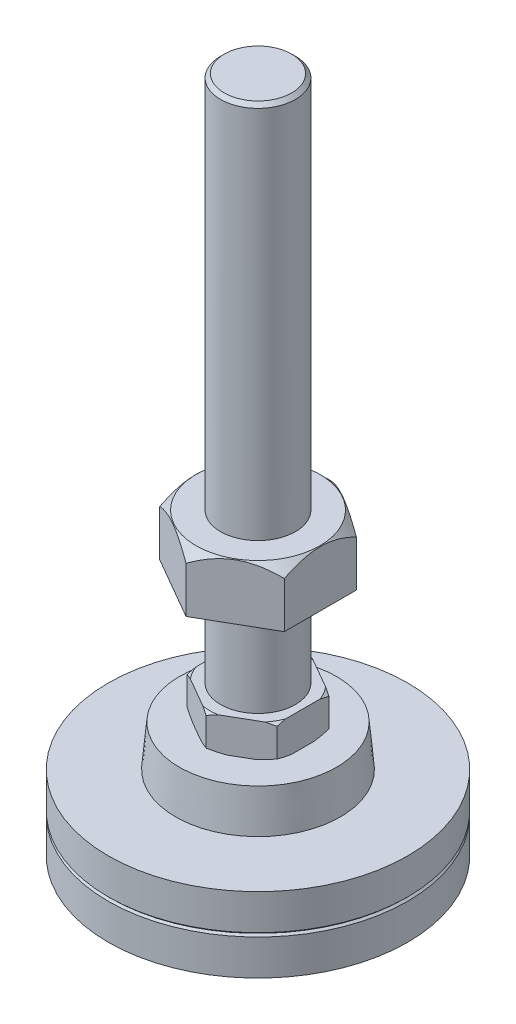
SolidWorks part; units mm, degrees
ref_plane "Front Plane" through (0, 0, 0) normal (0, 0, 1) x (1, 0, 0)
ref_plane "Top Plane" through (0, 0, 0) normal (0, 1, 0) x (1, 0, 0)
ref_plane "Right Plane" through (0, 0, 0) normal (1, 0, 0) x (0, 0, -1)
sketch "Sketch1" plane through (0, 0, 0) normal (0, 0, 1) x (1, 0, 0)
  line L0 (15, 0) -> (40, 0)
  line L1 (40, 0) -> (40, 9.5)
  line L2 (40, 20) -> (22, 20)
  line L3 (22, 20) -> (21, 31)
  line L4 (21, 31) -> (10, 31)
  line L5 (10, 31) -> (10, 181)
  line L6 (10, 181) -> (0, 181)
  line L7 (0, 181) -> (0, 15)
  line L8 (40, 10) -> (59.189, 10) construction
  line L9 (40, 10.5) -> (39.5, 10)
  line L10 (39.5, 10) -> (40, 9.5)
  line L11 (0, 15) -> (14, 15)
  line L12 (14, 15) -> (15, 0)
  line L13 (66, 0) -> (-66, 0) construction
  line L14 (40, 10.5) -> (40, 20)
  line L15 (0, 15) -> (0, 0) construction
  point P0 (5, 181)
  dimension "D1" = 20
  dimension "D2" = 181
  dimension "D3" = 10
  dimension "D4" = 11
  dimension "D5" = 31
  dimension "D6" = 18
  dimension "D7" = 40
  dimension "D8" = 10
  dimension "D9" = 0.5
  dimension "D10" = 1
  dimension "D11" = 0.5
  dimension "D12" = 15
  dimension "D13" = 25
  dimension "D14" = 14
  dimension "D15" = 45
revolve "Revolve1" add sketch "Sketch1" angle 360 about L7
cosmetic thread "Cosmetic Thread1" parameters "D2"=19
sketch "Sketch2" plane through (0, 31, 0) normal (0, 1, 0) x (1, 0, 0)
  line L1 (12, 6.9282) -> (0, 13.8564)
  line L2 (0, 13.8564) -> (-12, 6.9282)
  line L3 (-12, 6.9282) -> (-12, -6.9282)
  line L4 (-12, -6.9282) -> (0, -13.8564)
  line L5 (0, -13.8564) -> (12, -6.9282)
  line L6 (12, -6.9282) -> (12, 6.9282)
  circle A0 centre (0, 0) radius 12 construction
  dimension "D1" = 24
extrude "Boss-Extrude1" add sketch "Sketch2" along normal blind 9
sketch "Sketch3" plane through (0, 0, 0) normal (1, 0, 0) x (0, 0, -1)
  line L0 (12.3564, 31) -> (13.8564, 31.866)
  line L1 (6.9282, 31) -> (13.8564, 31) construction
  line L2 (13.8564, 40) -> (13.8564, 31) construction
  line L3 (13.8564, 31.866) -> (13.8564, 31)
  line L4 (13.8564, 39.4226) -> (12.8564, 40)
  line L5 (6.9282, 40) -> (13.8564, 40) construction
  line L6 (12.8564, 40) -> (13.8564, 40)
  line L7 (13.8564, 40) -> (13.8564, 39.4226)
  line L8 (21, 31) -> (-21, 31) construction
  line L9 (13.8564, 31) -> (12.3564, 31)
  dimension "D1" = 30
  dimension "D2" = 1.5
  dimension "D3" = 30
  dimension "D4" = 1
revolve "Cut-Revolve1" cut sketch "Sketch3" angle 360 about axis through (0, 181, 0) along (0, 1, 0)
ref_plane "Plane1" through (0, 41, 0) normal (0, 1, 0) x (-1, 0, 0)
sketch "Sketch5" plane through (0, 41, 0) normal (0, 1, 0) x (-1, 0, 0)
  line L1 (0, 19.2258) -> (-16.65, 9.6129)
  line L2 (-16.65, 9.6129) -> (-16.65, -9.6129)
  line L3 (-16.65, -9.6129) -> (0, -19.2258)
  line L4 (0, -19.2258) -> (16.65, -9.6129)
  line L5 (16.65, -9.6129) -> (16.65, 9.6129)
  line L6 (16.65, 9.6129) -> (0, 19.2258)
  circle A0 centre (0, 0) radius 16.65 construction
  circle A1 centre (0, 0) radius 10
  dimension "D1" = 33.3
  dimension "D2" = 20
extrude "Boss-Extrude2" add sketch "Sketch5" along normal blind 15 from offset 24
sketch "Sketch7" plane through (0, 0, 0) normal (1, 0, 0) x (0, 0, -1)
  line L0 (16.5258, 80) -> (19.2258, 77.3)
  line L1 (9.6129, 80) -> (19.2258, 80) construction
  line L2 (19.2258, 80) -> (19.2258, 65) construction
  line L3 (19.2258, 77.3) -> (19.2258, 80)
  line L4 (19.2258, 80) -> (16.5258, 80)
  line L5 (16.5258, 41) -> (19.2258, 43.7)
  line L6 (23.1, 41) -> (-23.1, 41) construction
  line L7 (19.2258, 43.7) -> (19.2258, 41)
  line L8 (19.2258, 41) -> (16.5258, 41)
  dimension "D1" = 45
  dimension "D2" = 2.7
  dimension "D3" = 2.7
  dimension "D4" = 45
revolve "Cut-Revolve3" cut sketch "Sketch7" angle 360 about axis through (0, 181, 0) along (0, 1, 0)
chamfer "Chamfer1" distance 1 angle 45 1 edges at (-10, 181, 0)
